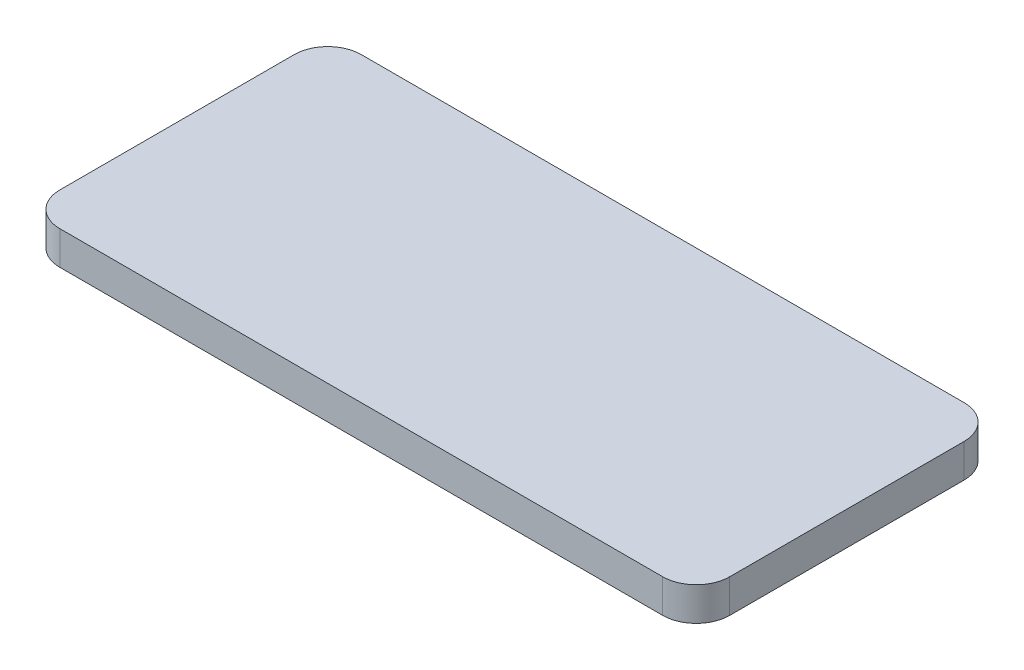
SolidWorks part; units mm, degrees
ref_plane "Front Plane" through (0, 0, 0) normal (0, 0, 1) x (1, 0, 0)
ref_plane "Top Plane" through (0, 0, 0) normal (0, 1, 0) x (1, 0, 0)
ref_plane "Right Plane" through (0, 0, 0) normal (1, 0, 0) x (0, 0, -1)
sketch "Sketch1" plane through (0, 0, 0) normal (0, 1, 0) x (1, 0, 0)
  line L1 (0, 0) -> (200, 0)
  line L2 (0, 0) -> (0, 90)
  line L3 (0, 90) -> (200, 90)
  line L4 (200, 0) -> (200, 90)
  dimension "D1" = 200
  dimension "D2" = 90
extrude "Boss-Extrude1" add sketch "Sketch1" along normal blind 10
fillet "Fillet1" radius 10 4 edges at (0, 5, -90) (0, 5, 0) (200, 5, -90) (200, 5, 0)
